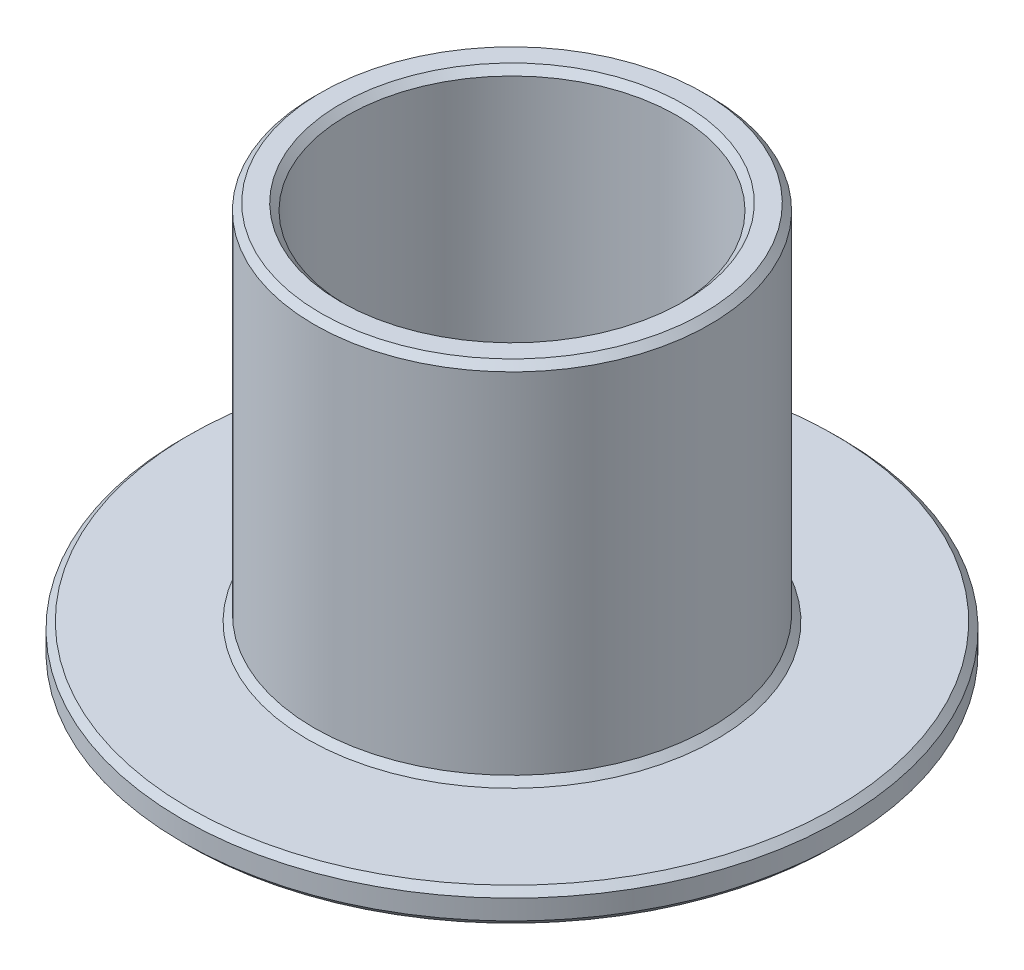
from build123d import *

# Parameters (mm, degrees)
CHAMFER_1_SIZE = 0.1


with BuildPart() as part:
    # 草图1 → 旋转1 (revolve)
    with BuildSketch(Plane.XY, mode=Mode.PRIVATE) as revolve_1_sk:
        Polygon((2.5, 0), (5, 0), (5, 0.5), (3, 0.5), (3, 6), (2.5, 6), align=None)
    revolve(revolve_1_sk.sketch.rotate(Axis((0, 0, 0), (0, 1, 0)), 90), axis=Axis((0, 0, 0), (0, 1, 0)))

    # 倒角1
    chamfer_1_edges = [part.edges().sort_by_distance(p)[0] for p in [
        (0, 6, 2.5),
        (0, 6, 3),
        (0, 0.5, 3),
        (0, 0.5, 5),
        (0, 0, 5),
        (0, 0, 2.5),
    ]]
    chamfer(chamfer_1_edges, length=CHAMFER_1_SIZE)


solid = part.part
